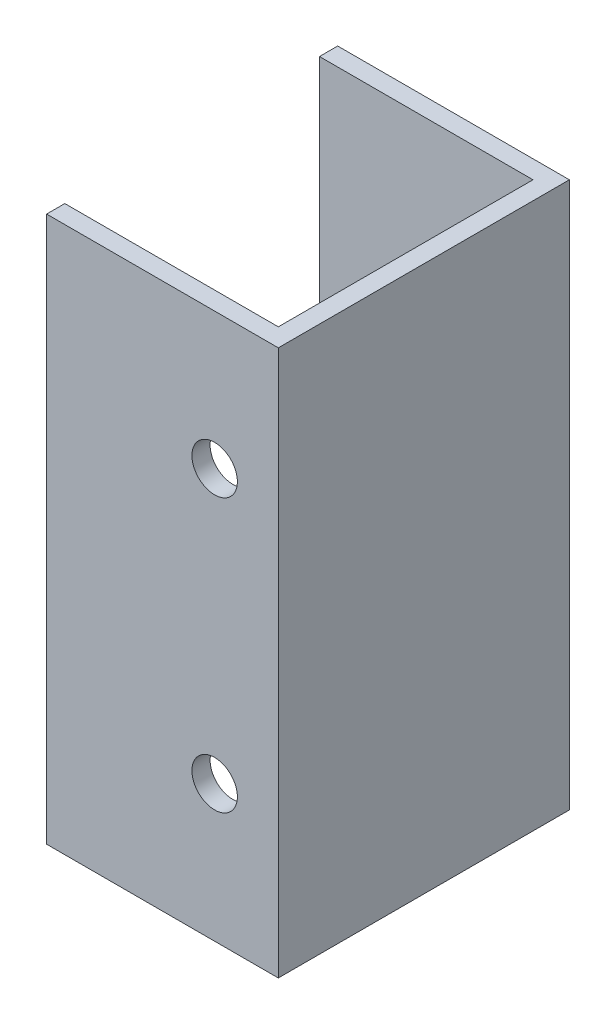
from build123d import *

# Parameters (mm, degrees)
BOSS_EXTRUDE1_DEPTH      = 30
BOSS_EXTRUDE1_DEPTH_BACK = 30
SKETCH3_R                = 2.5
CUT_EXTRUDE1_DEPTH       = 96.420123664


with BuildPart() as part:
    # Sketch2 → Boss-Extrude1 (new, two sides: drawn at the far end of the back side and taken through both)
    with BuildSketch(Plane(origin=(0, 50, 0), x_dir=(-1, 0, 0), z_dir=(0, -1, 0)).offset(-BOSS_EXTRUDE1_DEPTH_BACK)):
        Polygon((-39, 28), (-15.526318688, 28), (-15.526318688, 30), (-41, 30), (-41, -2), (-15.526318688, -2), (-15.526318688, 0), (-39, 0), align=None)
    extrude(amount=BOSS_EXTRUDE1_DEPTH + BOSS_EXTRUDE1_DEPTH_BACK)

    # Sketch3 → Cut-Extrude1 (cut, symmetric)
    with BuildSketch(Plane.XY.offset(2)):
        with Locations((34, 65)):
            Circle(SKETCH3_R)
    cut_extrude1 = extrude(amount=CUT_EXTRUDE1_DEPTH, both=True, mode=Mode.SUBTRACT)

    # Mirror1: Cut-Extrude1 across plane
    add(cut_extrude1.mirror(Plane(origin=(0, 50, 0), x_dir=(0, 0, 1), z_dir=(0, -1, 0))), mode=Mode.SUBTRACT)


solid = part.part
